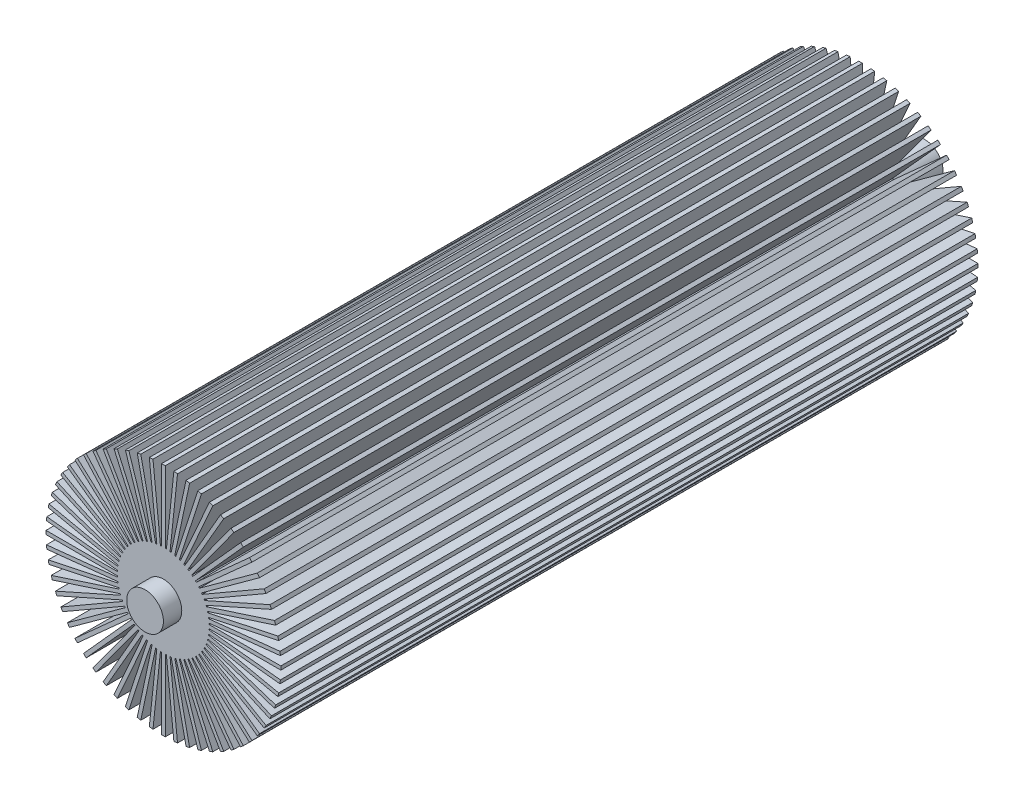
SolidWorks part; units mm, degrees
ref_plane "前视基准面" through (0, 0, 0) normal (0, 0, 1) x (1, 0, 0)
ref_plane "上视基准面" through (0, 0, 0) normal (0, 1, 0) x (1, 0, 0)
ref_plane "右视基准面" through (0, 0, 0) normal (1, 0, 0) x (0, 0, -1)
sketch "草图1" plane through (0, 0, 0) normal (0, 0, 1) x (1, 0, 0)
  circle A0 centre (0, 0) radius 25
  dimension "D1" = 50
extrude "凸台-拉伸1" add sketch "草图1" along normal blind 380
sketch "草图2" plane through (0, 0, 380) normal (0, 0, 1) x (1, 0, 0)
  circle A0 centre (0, 0) radius 10
  dimension "D1" = 20
extrude "凸台-拉伸2" add sketch "草图2" along normal blind 10
sketch "草图3" plane through (0, 0, 0) normal (0, 0, -1) x (-1, 0, 0)
  circle A0 centre (0, 0) radius 10
  dimension "D1" = 20
extrude "凸台-拉伸3" add sketch "草图3" along normal blind 35
sketch "草图4" plane through (0, 0, 0) normal (0, 0, -1) x (-1, 0, 0)
  line L0 (0, 0) -> (0, 25) construction
  line L1 (0, 0) -> (31.3318, 0) construction
  line L2 (-1, 24) -> (1, 24)
  line L3 (-1, 24) -> (-1, 64)
  line L4 (-1, 64) -> (1, 64)
  line L5 (1, 24) -> (1, 64)
  circle A0 centre (0, 0) radius 25 construction
  dimension "D1" = 24
  dimension "D2" = 2
  dimension "D3" = 40
extrude "凸台-拉伸4" add sketch "草图4" against normal up to surface (380 mm away) up to face at (10, 0, 380)
pattern_circular "阵列(圆周)1" count 60 over 360 about axis through (0, 0, 0) along (0, 0, 1) of "凸台-拉伸4"
